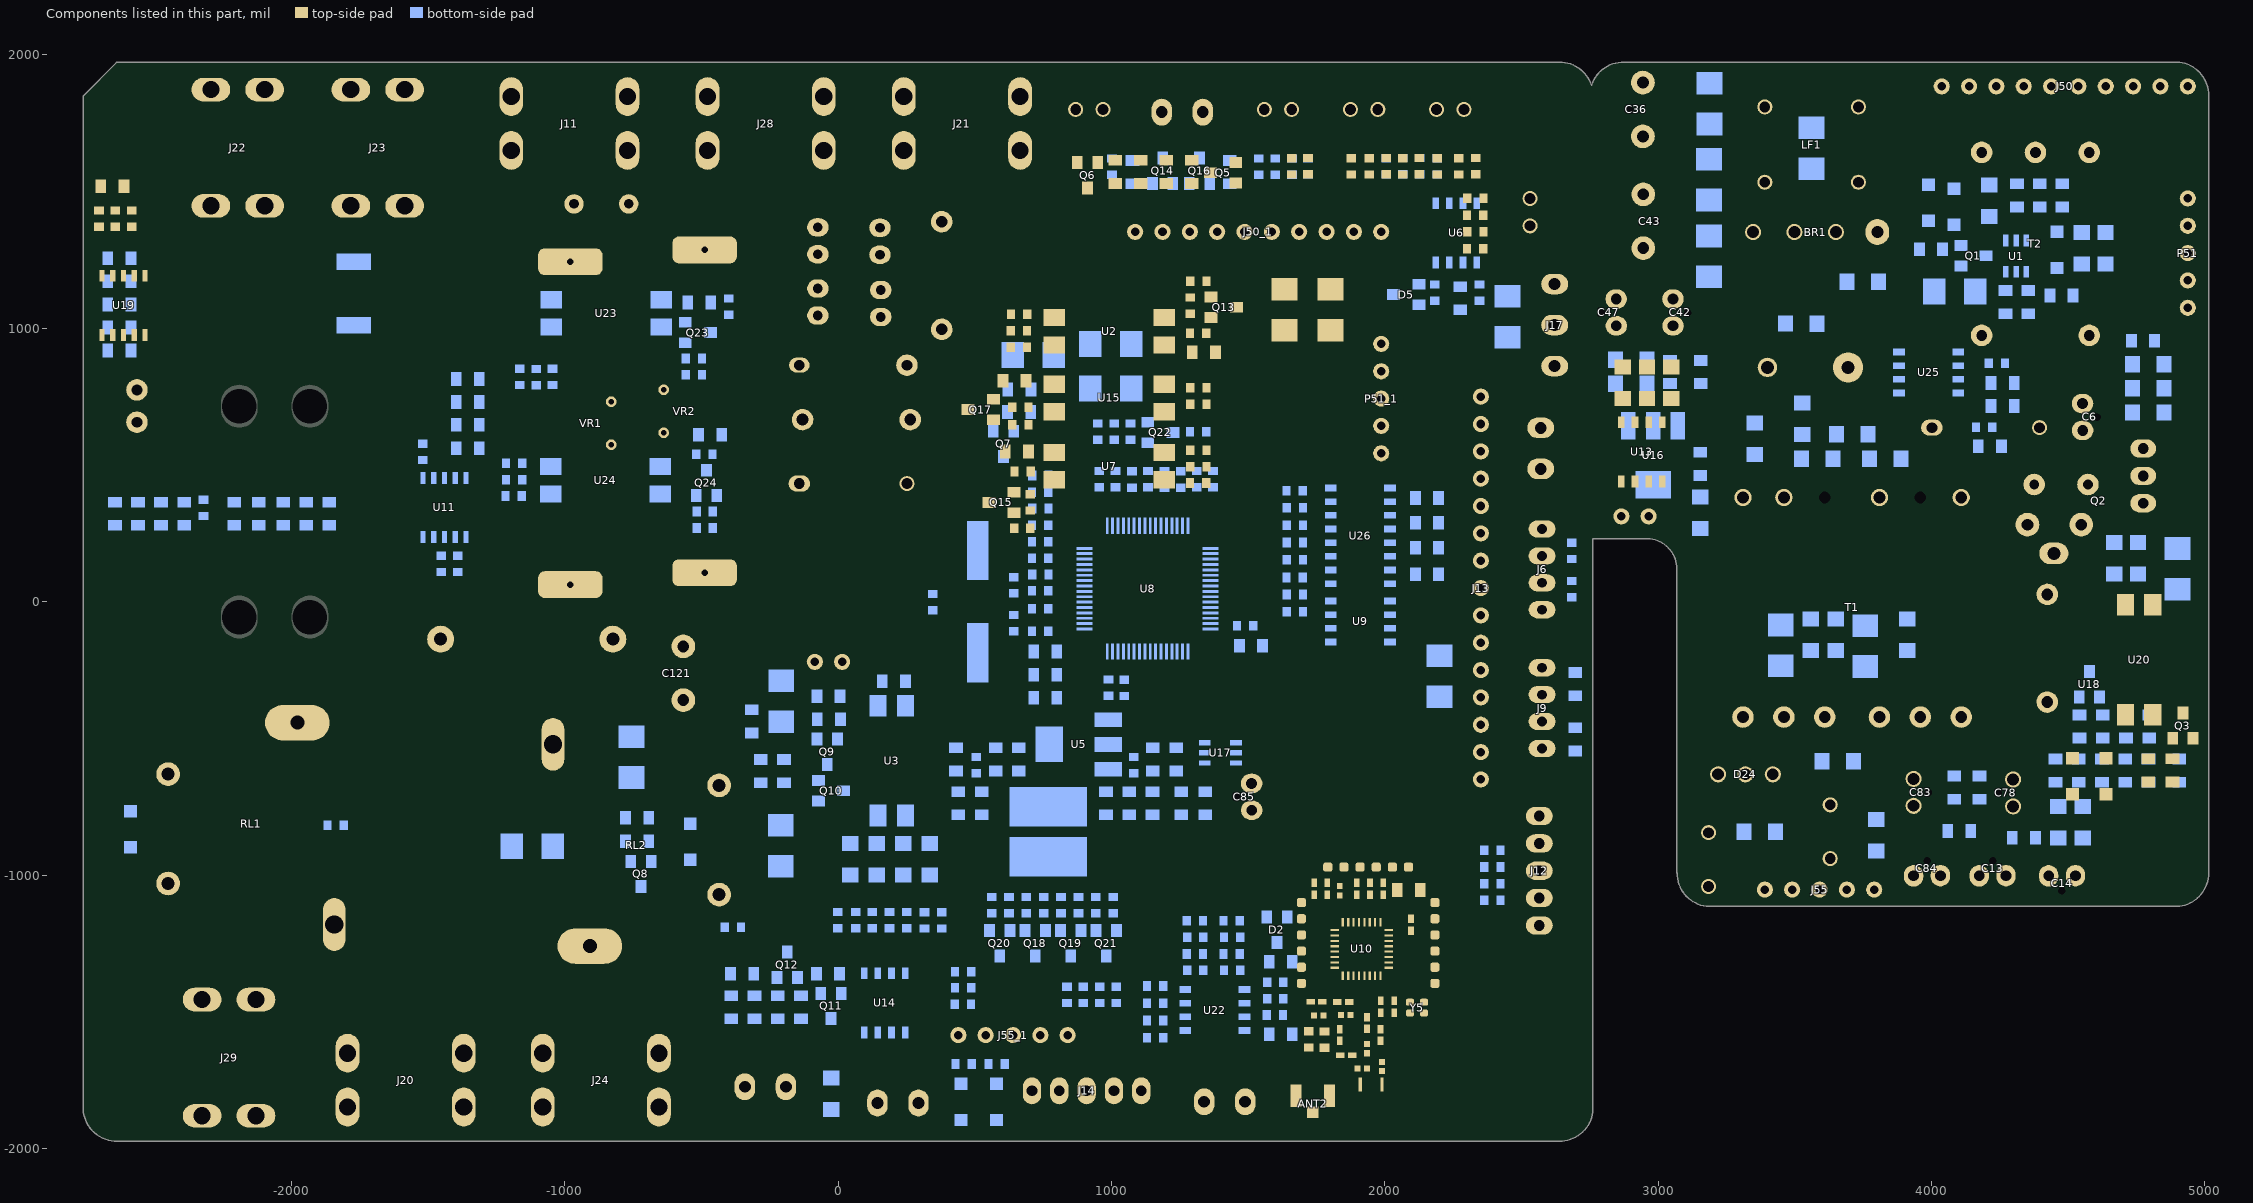
[diagram p0: the components of this part, seen from the top]
# Altium PCB MISC105418.PcbDoc (part 7 of 7)
Units mil, origin at the board's own origin, x right, y up, seen from the top; angles counter-clockwise.
Board outline 7774.32 x 3947.04 mil, 4 copper layers (Top Layer, 02, 03, Bottom Layer), stack 30.635 mil thick; 459 components, 285 nets, 1258 pads, 468 vias.
Unrouted connection lines stored in the file: 23.

## Polygon pours and split planes (outlines as drawn) (continued)
NetJP1_2 on Bottom Layer "NETJP1_2_L04_P172" (solid, remove dead copper, pour order 172): -2541,-310 -2257,-594 -1889,-594 -1857,-562 -1857,-403 -1888,-372 -2080,-372 -2121,-331 -2121,55 -2168,102 -2483,102 -2541,44
NetJP2_2 on Bottom Layer "NETJP2_2_L04_P170" (solid, remove dead copper, pour order 170): -2007,56 -2007,-198 -1950,-255 -1848,-255 -1727,-376 -1727,-585 -1651.67,-660.32 -1008.58,-660.33 -965,-616.74 -965,-433 -1084.99,-313 -1511,-313 -1632,-192 -1632,59 -1677,104 -1959,104
N2 on Bottom Layer "N2_L04_P198" (solid, remove dead copper, pour order 198): -534,1897 -534,1396 -610,1320 -610,1244 -597,1231 -353,1231 -248,1336 -37,1336 -6,1367 -6,1897 -39,1930 -501,1930
L-PLC on Bottom Layer "L-PLC_L04_P184" (solid, remove dead copper, pour order 184): -1193.8,1253.8 -1164,1224 -953,1224 -925,1252 -925,1464 -950,1489 -1168.58,1489 -1193.8,1462.76
L2 on Bottom Layer "L2_L04_P174" (solid, remove dead copper, pour order 174): -804,1389 -804,1534 -827,1557 -1240,1557 -1283,1600 -1283,1890 -1237,1936 -711,1936 -698,1923 -698,1387 -712,1373 -788,1373
ACL-OUT on Bottom Layer "ACL-OUT_L04_P146" (solid, remove dead copper, pour order 146): -1824,-1945 -1872,-1897 -1872,-1333 -1948,-1257 -1948,-1049 -1888,-989 -1394,-989 -1294,-1089 -1294,-1934 -1305,-1945
IP2 on Bottom Layer "IP2_L04_P132" (solid, remove dead copper, pour order 132): -1660,611 -1626,645 -1626,986 -1689,1049 -1803,1049 -2003,849 -2003,635 -1979,611
ACN-IN on Bottom Layer "ACN-IN_L04_P118" (solid, remove dead copper, pour order 118): -1552,1196 -1482,1266 -1482,1901 -1530,1949 -1839,1949 -1880,1908 -1880,1253 -1823,1196
ACN-OUT on Bottom Layer "ACN-OUT_L04_P116" (solid, remove dead copper, pour order 116): -1073,-1187 -1168,-1282 -1168,-1892 -1111,-1949 -620,-1949 -572,-1901 -572,-1275 -660,-1187
NetVR1_1 on Bottom Layer "NETVR1_1_L04_P044" (solid, remove dead copper, pour order 44): -1043,-198 -816,-198 -575,43 -374,43 -352,65 -352,134.25 -383.75,166 -1155,166 -1177,144 -1177,-64
NetC7_1 on Bottom Layer "NETC7_1_L04_P006" (solid, remove dead copper, pour order 6): 4783,187 4559,187 4494,252 4494,452 4519,477 4578,477 4610,445 4610,301.36 4666.35,245 4784,245 4791,238 4791,195
EARTH on Bottom Layer "EARTH_L04_P301" (solid, remove dead copper, pour order 301): 169,1538 195,1512 298,1512 321,1489 321,1372 347,1346 461,1346 481,1366 481,1472 510,1501 686,1501 735,1550 735,1921 704,1952 191,1952 169,1930
- on Top Layer "-_L01_P345" (solid, remove dead copper, pour order 345): 935,1901 935,872 -378,-441 -378,-1853 -301,-1930 2598,-1930 2700,-1828 2700,1851 2625,1926 960,1926
- on Top Layer "-_L01_P341" (solid, remove dead copper, pour order 341): 1541,-1443 1541,-1872 1620,-1951 1837,-1951 1879,-1909 1879,-1746 1900,-1725 2265,-1725 2286,-1704 2286,-1463 2246,-1423 2245,-1424 1560,-1424
- on Top Layer "-_L01_P339" (solid, remove dead copper, pour order 339): 1846,-1233 1846,-1315 1853,-1322 1924,-1322 1934,-1312 1934,-1239 1920,-1225 1854,-1225
EARTH on Top Layer "EARTH_L01_P331" (solid, remove dead copper, pour order 331): 169,1538 195,1512 298,1512 321,1489 321,1372 347,1346 461,1346 481,1366 481,1472 510,1501 686,1501 735,1550 735,1921 704,1952 191,1952 169,1930
EARTH on Top Layer "EARTH_L01_P323" (solid, remove dead copper, pour order 323): -2082,-1921 -2379,-1921 -2409,-1891 -2409,-1444 -2370,-1405 -2090,-1405 -2059,-1436 -2059,-1898
NetCX1_1 on Top Layer "Top Layer-NetCX1_1" (solid, remove dead copper, pour order 280): -7,1236 91,1334 205,1334 265,1274 265,1041 111,887 111,464 185,390 269,390 287.68,408.68 287.68,453.32 266,475 204,475 157,522 157,880 228,951 396,951 422,977 422,1012 398,1036 336,1036 318,1054 318,1293 205,1406 110,1406 9,1305 -96,1305 -111,1290 -111,1250 -97,1236
NetCX1_2 on Top Layer "NETCX1_2_L01_P277" (solid, remove dead copper, pour order 277): -104,392 -91,405 -91,679 54,824 54,1064 94,1104 195,1104 206,1115 206,1174 197,1183 74,1183 -28,1081 -97,1081 -122,1056 -122,1025 -45,948 -45,840 -192,693 -192,404 -180,392
L-3 on Top Layer "L-3_L01_P254" (solid, remove dead copper, pour order 254): 3406,1773 3511,1878 3950,1878 3982,1846 4061,1846 4073,1858 4073,1912 4050,1935 3435.74,1935 3352,1851.26 3352,1794 3373,1773
N on Top Layer "N_L01_P246" (solid, remove dead copper, pour order 246): 2827,1079 2879,1079 3012,1212 3620,1212 3696,1288 3696,1434 3769,1507 3769,1542 3746,1565 3719,1565 3617,1463 3617,1336 3571,1290 3034,1290 3006,1290 2862,1434 2862,1771 2905,1814 2940,1814 3001,1875 3001,1921 2978,1944 2856,1944 2811,1899 2811,1095
N2 on Top Layer "N2_L01_P234" (solid, remove dead copper, pour order 234): 4618,937 4788,1107 4788,1768 4644,1912 4626,1912 4613,1899 4613,1865 4739,1739 4739,1134 4616,1011 4561,1011 4539,989 4539,962 4564,937
NetCX3_1 on Top Layer "NETCX3_1_L01_P232" (solid, remove dead copper, pour order 232): 4148,723 4262,609 4413,609 4426,622 4426,647.39 4408.2,665.2 4293.8,665.2 4216,743 4216,993 4202,1007 4168.95,1007 4148,986.05
+311V on Top Layer "+311V_L01_P228" (solid, remove dead copper, pour order 228): 3758,1377 3758,1086 3635,963 3635,716 3926,425 4126,225 4370,225 4426,281 4426,433 4395,464 4004,464 3758.01,710 3758,953.34 3849,1044.34 3849,1381 3836.99,1393 3774,1393
NetJP2_2 on Top Layer "NETJP2_2_L01_P210" (solid, remove dead copper, pour order 210): -2007,56 -2007,-198 -1950,-255 -1848,-255 -1727,-376 -1727,-585 -1651.67,-660.32 -1008.58,-660.33 -965,-616.74 -965,-433 -1084.99,-313 -1511,-313 -1632,-192 -1632,59 -1677,104 -1959,104
NetJP1_2 on Top Layer "NETJP1_2_L01_P208" (solid, remove dead copper, pour order 208): -2541,-310 -2257,-594 -1889,-594 -1857,-562 -1857,-403 -1888,-372 -2080,-372 -2121,-331 -2121,55 -2168,102 -2483,102 -2541,44
NetVR1_1 on Top Layer "NETVR1_1_L01_P202" (solid, remove dead copper, pour order 202): -1043,-198 -824,-198 -605,21 -405,21 -345,81 -345,266 -398.01,319 -1105,319 -1177,247 -1177,-64
L2 on Top Layer "L2_L01_P176" (solid, remove dead copper, pour order 176): -804,1389 -804,1534 -827,1557 -1240,1557 -1283,1600 -1283,1890 -1237,1936 -711,1936 -698,1923 -698,1387 -712,1373 -788,1373
ACN-OUT on Top Layer "ACN-OUT_L01_P156" (solid, remove dead copper, pour order 156): -1073,-1187 -1168,-1282 -1168,-1892 -1111,-1949 -620,-1949 -572,-1901 -572,-1275 -660,-1187
ACL-OUT on Top Layer "ACL-OUT_L01_P154" (solid, remove dead copper, pour order 154): -1824,-1945 -1872,-1897 -1872,-1333 -1948,-1257 -1948,-1049 -1888,-989 -1394,-989 -1294,-1089 -1294,-1934 -1305,-1945
IP2 on Top Layer "IP2_L01_P138" (solid, remove dead copper, pour order 138): -1660,611 -1626,645 -1626,986 -1689,1049 -1798,1049 -2003,844 -2003,635 -1979,611
ACN-IN on Top Layer "ACN-IN_L01_P126" (solid, remove dead copper, pour order 126): -1552,1196 -1482,1266 -1482,1901 -1530,1949 -1839,1949 -1880,1908 -1880,1253 -1823,1196
ACL-IN on Top Layer "ACL-IN_L01_P120" (solid, remove dead copper, pour order 120): -2374,1900 -2374,1369 -2309,1304 -2309,665.39 -2281.61,638 -2154,638 -2127,665 -2127,901 -2003,1025 -2003,1892 -2050,1939 -2335,1939
L-PLC on Top Layer "L-PLC_L01_P291" (solid, remove dead copper, pour order 291): -1193.8,1253.8 -1164,1224 -953,1224 -925,1252 -925,1464 -950,1489 -1168.58,1489 -1193.8,1462.76
N2 on Top Layer "N2_L01_P293" (solid, remove dead copper, pour order 293): -534,1897 -534,1396 -610,1320 -610,1244 -597,1231 -353,1231 -248,1336 -37,1336 -6,1367 -6,1897 -39,1930 -501,1930
L-PLC on Top Layer "L-PLC_L01_P311" (solid, remove dead copper, pour order 311): -995,1055 -198,1055 -143,1110 -50,1110 -29,1131 -29,1159 -50,1180 -205,1180 -241,1144 -815.2,1144 -964.2,1293 -1157,1293 -1182,1268 -1182,1242
- on 03 "-_L03_P347" (solid, remove dead copper, pour order 347): 935,1901 935,760 -378,-553 -378,-1853 -301,-1930 2598,-1930 2700,-1828 2700,1851 2625,1926 960,1926
EARTH on 03 "EARTH_L03_P337" (solid, remove dead copper, pour order 337): 169,1538 195,1512 298,1512 321,1489 321,1372 347,1346 461,1346 481,1366 481,1472 510,1501 686,1501 735,1550 735,1921 704,1952 191,1952 169,1930
EARTH on 03 "EARTH_L03_P327" (solid, remove dead copper, pour order 327): -2082,-1921 -2379,-1921 -2409,-1891 -2409,-1444 -2370,-1405 -2090,-1405 -2059,-1436 -2059,-1898
L-3 on 03 "L-3_L03_P307" (solid, remove dead copper, pour order 307): 130,1061 130,920 228,822 731,822 1132,1223 1132,1379 1110,1401 1057.74,1401 1032,1375.26 1032,1249 706,923 623,923 288,923 235,976 235,1049 208,1076 145,1076
N-3 on 03 "N-3_L03_P305" (solid, remove dead copper, pour order 305): 42,823 77,858 77,1175 136,1234 224,1234 304,1154 810,1154 911,1255 911,1498 956,1543 1192,1543 1242,1493 1242,1310 1267,1285 1314,1285 1339,1310 1339,1524.86 1255.86,1608 898,1608 830,1540 830,1330 753,1253 326,1253 254,1325 115,1325 3,1213 3,982 -53,926 -199,926 -215,910 -215,839 -199,823
GND on 03 "03-GND" (solid, remove dead copper, pour order 270): 3236,275 3334,177 4084,177 4314,-53 4538,-53 4622,31 4622,497 4758,633 4758,1316.02 4484,1590 3963,1590 3808,1435 3319,1435 3236,1352
- on 03 "-_L03_P260" (solid, remove dead copper, pour order 260): 3955,-33 4147,-225 4845,-225 4974,-354 4974,-960 4858,-1076 3202.2,-1076 3105.2,-979 3105.2,-67.8 3140,-33
NetJP2_2 on 03 "NETJP2_2_L03_P214" (solid, remove dead copper, pour order 214): -2007,56 -2007,-198 -1950,-255 -1848,-255 -1727,-376 -1727,-585 -1651.67,-660.32 -1008.58,-660.33 -965,-616.74 -965,-433 -1084.99,-313 -1511,-313 -1632,-192 -1632,59 -1677,104 -1959,104
NetJP1_2 on 03 "NETJP1_2_L03_P212" (solid, remove dead copper, pour order 212): -2541,-310 -2257,-594 -1889,-594 -1857,-562 -1857,-403 -1888,-372 -2080,-372 -2121,-331 -2121,55 -2168,102 -2483,102 -2541,44
L2 on 03 "L2_L03_P180" (solid, remove dead copper, pour order 180): -804,1389 -804,1534 -827,1557 -1240,1557 -1283,1600 -1283,1890 -1237,1936 -711,1936 -698,1923 -698,1387 -712,1373 -788,1373
ACN-OUT on 03 "ACN-OUT_L03_P164" (solid, remove dead copper, pour order 164): -1073,-1187 -1168,-1282 -1168,-1892 -1111,-1949 -620,-1949 -572,-1901 -572,-1275 -660,-1187
ACL-OUT on 03 "ACL-OUT_L03_P162" (solid, remove dead copper, pour order 162): -1824,-1945 -1872,-1897 -1872,-1333 -1948,-1257 -1948,-1049 -1888,-989 -1394,-989 -1294,-1089 -1294,-1934 -1305,-1945
IP2 on 03 "IP2_L03_P134" (solid, remove dead copper, pour order 134): -1660,611 -1626,645 -1626,986 -1689,1049 -1798,1049 -2003,844 -2003,635 -1979,611
ACL-IN on 03 "ACL-IN_L03_P130" (solid, remove dead copper, pour order 130): -2374,1900 -2374,1369 -2309,1304 -2309,665.39 -2281.61,638 -2154,638 -2127,665 -2127,901 -2003,1025 -2003,1892 -2050,1939 -2335,1939
ACN-IN on 03 "ACN-IN_L03_P128" (solid, remove dead copper, pour order 128): -1552,1196 -1482,1266 -1482,1901 -1530,1949 -1839,1949 -1880,1908 -1880,1253 -1823,1196
L-PLC on 03 "L-PLC_L03_P283" (solid, remove dead copper, pour order 283): -1193.8,1253.8 -1164,1224 -953,1224 -925,1252 -925,1464 -950,1489 -1168.58,1489 -1193.8,1462.76
N2 on 03 "N2_L03_P285" (solid, remove dead copper, pour order 285): -534,1897 -534,1396 -610,1320 -610,1244 -597,1231 -353,1231 -248,1336 -37,1336 -6,1367 -6,1897 -39,1930 -501,1930
NetVR1_1 on 03 "NETVR1_1_L03_P297" (solid, remove dead copper, pour order 297): -1043,-198 -824,-198 -605,21 -405,21 -345,81 -345,266 -398.01,319 -1105,319 -1177,247 -1177,-64
- on 02 "-_L02_P349" (solid, remove dead copper, pour order 349): -993,625 -963,595 -827,595 -692,730 -408,730 -325,813 -325,999 -396,1070 -911,1070 -993,988
- on 02 "-_L02_P343" (solid, remove dead copper, pour order 343): 935,1901 935,760 -378,-553 -378,-1853 -301,-1930 2598,-1930 2700,-1828 2700,1851 2625,1926 960,1926
EARTH on 02 "EARTH_L02_P335" (solid, remove dead copper, pour order 335): 169,1538 195,1512 298,1512 321,1489 321,1372 347,1346 461,1346 481,1366 481,1472 510,1501 686,1501 735,1550 735,1921 704,1952 191,1952 169,1930
EARTH on 02 "EARTH_L02_P325" (solid, remove dead copper, pour order 325): -2082,-1921 -2379,-1921 -2409,-1891 -2409,-1444 -2370,-1405 -2090,-1405 -2059,-1436 -2059,-1898
NetJP2_2 on 02 "NETJP2_2_L02_P222" (solid, remove dead copper, pour order 222): -2007,56 -2007,-198 -1950,-255 -1848,-255 -1727,-376 -1727,-585 -1651.67,-660.32 -1008.58,-660.33 -965,-616.74 -965,-433 -1084.99,-313 -1511,-313 -1632,-192 -1632,59 -1677,104 -1959,104
NetJP1_2 on 02 "NETJP1_2_L02_P220" (solid, remove dead copper, pour order 220): -2541,-310 -2257,-594 -1889,-594 -1857,-562 -1857,-403 -1888,-372 -2080,-372 -2121,-331 -2121,55 -2168,102 -2483,102 -2541,44
GND on 02 "02-GND" (solid, remove dead copper, pour order 271): 3236,275 3334,177 4084,177 4314,-53 4538,-53 4622,31 4622,497 4758,633 4758,911 4198,1471 4109,1560 3933,1560 3808,1435 3319,1435 3236,1352
- on 02 "-_L02_P262" (solid, remove dead copper, pour order 262): 3955,-33 4147,-225 4845,-225 4974,-354 4974,-960 4858,-1076 3202.2,-1076 3105.2,-979 3105.2,-67.8 3140,-33
L2 on 02 "L2_L02_P178" (solid, remove dead copper, pour order 178): -804,1389 -804,1534 -827,1557 -1240,1557 -1283,1600 -1283,1890 -1237,1936 -711,1936 -698,1923 -698,1387 -712,1373 -788,1373
ACN-OUT on 02 "ACN-OUT_L02_P160" (solid, remove dead copper, pour order 160): -1073,-1187 -1168,-1282 -1168,-1892 -1111,-1949 -620,-1949 -572,-1901 -572,-1275 -660,-1187
ACL-OUT on 02 "ACL-OUT_L02_P158" (solid, remove dead copper, pour order 158): -1824,-1945 -1872,-1897 -1872,-1333 -1948,-1257 -1948,-1049 -1888,-989 -1394,-989 -1294,-1089 -1294,-1934 -1305,-1945
ACN-IN on 02 "ACN-IN_L02_P140" (solid, remove dead copper, pour order 140): -1552,1196 -1482,1266 -1482,1901 -1530,1949 -1839,1949 -1880,1908 -1880,1253 -1823,1196
IP2 on 02 "IP2_L02_P136" (solid, remove dead copper, pour order 136): -1660,611 -1626,645 -1626,986 -1689,1049 -1798,1049 -2003,844 -2003,635 -1979,611
ACL-IN on 02 "ACL-IN_L02_P122" (solid, remove dead copper, pour order 122): -2382,1902 -2382,1371 -2317,1306 -2317,667.39 -2289.61,640 -2162,640 -2135,667 -2135,903 -2011,1027 -2011,1894 -2058,1941 -2343,1941
L-PLC on 02 "L-PLC_L02_P287" (solid, remove dead copper, pour order 287): -1193.8,1253.8 -1164,1224 -953,1224 -925,1252 -925,1464 -950,1489 -1168.58,1489 -1193.8,1462.76
N2 on 02 "N2_L02_P289" (solid, remove dead copper, pour order 289): -534,1897 -534,1396 -610,1320 -610,1244 -597,1231 -353,1231 -248,1336 -37,1336 -6,1367 -6,1897 -39,1930 -501,1930
NetVR1_1 on 02 "NETVR1_1_L02_P295" (solid, remove dead copper, pour order 295): -1043,-198 -824,-198 -605,21 -405,21 -345,81 -345,266 -398.01,319 -1105,319 -1177,247 -1177,-64
ACL-OUT on Bottom Solder "ACL-OUT_L02_P158" (solid): -1824,-1945 -1872,-1897 -1872,-1333 -1948,-1257 -1948,-1049 -1888,-989 -1394,-989 -1294,-1089 -1294,-1934 -1305,-1945
ACN-OUT on Bottom Solder "ACN-OUT_L02_P160" (solid): -1073,-1187 -1168,-1282 -1168,-1892 -1111,-1949 -620,-1949 -572,-1901 -572,-1275 -660,-1187
EARTH on Bottom Solder "EARTH_L02_P325" (solid): -2082,-1921 -2379,-1921 -2409,-1891 -2409,-1444 -2370,-1405 -2090,-1405 -2059,-1436 -2059,-1898
NetVR1_1 on Bottom Solder "NETVR1_1_L04_P044" (solid): -1043,-198 -816,-198 -575,43 -374,43 -352,65 -352,134.25 -383.75,166 -1155,166 -1177,144 -1177,-64
NetJP2_2 on Bottom Solder "NETJP2_2_L04_P170" (solid): -2007,56 -2007,-198 -1950,-255 -1848,-255 -1727,-376 -1727,-585 -1651.67,-660.32 -1008.58,-660.33 -965,-616.74 -965,-433 -1084.99,-313 -1511,-313 -1632,-192 -1632,59 -1677,104 -1959,104
NetJP1_2 on Bottom Solder "NETJP1_2_L04_P172" (solid): -2541,-310 -2257,-594 -1889,-594 -1857,-562 -1857,-403 -1888,-372 -2080,-372 -2121,-331 -2121,55 -2168,102 -2483,102 -2541,44
ACN-IN on Bottom Solder "ACN-IN_L04_P118" (solid): -1552,1196 -1482,1266 -1482,1901 -1530,1949 -1839,1949 -1880,1908 -1880,1253 -1823,1196
IP2 on Bottom Solder "IP2_L04_P132" (solid): -1660,611 -1626,645 -1626,986 -1689,1049 -1803,1049 -2003,849 -2003,635 -1979,611
L2 on Bottom Solder "L2_L04_P174" (solid): -804,1389 -804,1534 -827,1557 -1240,1557 -1283,1600 -1283,1890 -1237,1936 -711,1936 -698,1923 -698,1387 -712,1373 -788,1373
L-PLC on Bottom Solder "L-PLC_L04_P184" (solid): -1193.8,1253.8 -1164,1224 -953,1224 -925,1252 -925,1464 -950,1489 -1168.58,1489 -1193.8,1462.76
N2 on Bottom Solder "N2_L04_P198" (solid): -534,1897 -534,1396 -610,1320 -610,1244 -597,1231 -353,1231 -248,1336 -37,1336 -6,1367 -6,1897 -39,1930 -501,1930
ACL-IN on Bottom Solder "ACL-IN_L04_P224" (solid): -2382,1902 -2382,1371 -2382,687 -2330,635 -2157,635 -2135,657 -2135,903 -2011,1027 -2011,1894 -2058,1941 -2343,1941
EARTH on Bottom Solder "EARTH_L04_P301" (solid): 169,1538 195,1512 298,1512 321,1489 321,1372 347,1346 461,1346 481,1366 481,1472 510,1501 686,1501 735,1550 735,1921 704,1952 191,1952 169,1930

## Keep-outs
Keep-Out Layer:
  lines w7.87: 2756.09,234.5 2756.09,1859.5
  lines w10: -2637.91,-1968.5 2637.09,-1968.5 ccw(c2639.05,-1850.39) 2756.09,-1866.21 2756.09,1859.5 ; -2636.91,-1968.49 cw(c-2638.86,-1850.39) -2755.91,-1866.21 -2755.91,1847.97 -2636.53,1968.5 2637.91,1968.5 ; 2636.91,1968.49 cw(c2638.86,1850.39) 2755.91,1866.21 ; 2755.91,-1859.5 2755.91,1866.21 ; 2756.09,235.5 2971.09,235.5 cw(c2955.28,118.46) 3073.37,116.5 ; 2874.91,1968.49 ccw(c2872.95,1850.39) 2755.91,1866.21 ; 2875.09,1968.5 4906.09,1968.5 cw(c4890.28,1851.46) 5008.37,1849.5 ; 3073.28,-990.5 3073.28,118.46 ; 3073.82,-990.5 ccw(c3191.91,-992.45) 3176.09,-1109.5 4906.09,-1109.5 ccw(c4890.28,-992.45) 5008.37,-990.5 ; 5007.98,-990.5 5007.98,1851.46
  lines w98.43: -2061.99,-207 -2062,82 ; -2061.99,568 -2062,857

## Other copper
Top Layer:
  pour cut-out: 2268,619 2286,601 2408,601 2431,624 2431,802 2402,831 2286,831 2268,813
  pour cut-out: 2006.98,1445 2046,1406.02 2046,1295.8 2011.21,1261.01 1086.75,1261 1061,1286.75 1061,1428 1078,1445
02:
  pour cut-out: -422.14,-850 -379,-850 -128,-1101 -128,-1930 -149,-1951 -174,-1926 -435,-1926 -465,-1896 -465,-1819
  pour cut-out: 3358,1448 3402,1404 3402,1300 3443,1259 3831,1259 3892,1320 3892,1529 3916,1553
  pour cut-out: 4296.35,428.5 ccw(c4375.09,428.5) 4375.09,349.76 ccw(c4375.09,428.5) 4453.83,428.5 ccw(c4375.09,428.5) 4375.09,507.24 ccw(c4375.09,428.5)
  pour cut-out: 4271.93,281.5 ccw(c4350.67,281.5) 4350.67,202.76 ccw(c4350.67,281.5) 4429.41,281.5 ccw(c4350.67,281.5) 4350.67,360.24 ccw(c4350.67,281.5)
  pour cut-out: 4029.57,381.08 ccw(c4108.31,381.08) 4108.31,302.34 ccw(c4108.31,381.08) 4187.05,381.08 ccw(c4108.31,381.08) 4108.31,459.82 ccw(c4108.31,381.08)
  pour cut-out: 3922.35,636.5 ccw(c4001.09,636.5) 4001.09,557.76 ccw(c4001.09,636.5) 4079.83,636.5 ccw(c4001.09,636.5) 4001.09,715.24 ccw(c4001.09,636.5)
  pour cut-out: 4497.96,974 ccw(c4576.7,974) 4576.7,895.26 ccw(c4576.7,974) 4655.44,974 ccw(c4576.7,974) 4576.7,1052.74 ccw(c4576.7,974)
  pour cut-out: 4104.26,974 ccw(c4183,974) 4183,895.26 ccw(c4183,974) 4261.74,974 ccw(c4183,974) 4183,1052.74 ccw(c4183,974)
  pour cut-out: 3615.9,857 ccw(c3694.64,857) 3694.64,778.26 ccw(c3694.64,857) 3773.38,857 ccw(c3694.64,857) 3694.64,935.74 ccw(c3694.64,857)
03:
  pour cut-out: 2041,1445 2046,1440 2046,1315.6 2011,1280.6 1379.48,1280.6 1347.2,1312.89 1347.2,1422.2 1370,1445
  pour cut-out: 1445,1282 926,763 916,763 916,959 1234,1277 1312.11,1277 1344.11,1309 1420,1309 1434,1295
  pour cut-out: 885,1657 1327,1657 1445,1539 1445,1282 1378.08,1282 1347.2,1312.89 1347.2,1520.8 1256,1612 899,1612 853,1658 853,1659
  pour cut-out: 3383,1447 3397,1433 3397,1297 3448,1246 3840,1246 3907.41,1313.41 3907.41,1534.59 3901,1541
Bottom Layer:
  rectangle net D5V: 626,-715 1091,-657
  rectangle net D5V: 416,-823 911,-744.83
  rectangle net D3.3V: 794,-553 1043,-491
  rectangle net D5V: 938,-715 1091,-630

## Silkscreen, mask and mechanical layers (free items; w line width, h text height)
Mechanical 6:
  circle w4.92: c-2598.43,1771.65 r98.43
  circle w4.92: c-2598.43,-1771.65 r98.43
  circle w4.92: c2598.43,-1771.65 r98.43
  circle w4.92: c2598.43,1771.65 r98.43
  lines w7.87: 887.81,-1534.74 890.81,-1537.74 ; 2756.09,234.5 2756.09,1859.5 ; 3838.09,-1002.5 3841.09,-1005.5 ; -194.19,-297.74 -194.19,1327.26 -194.19,-297.74 ; -134.28,-272.24 64.72,-272.24 64.72,-170.24 -134.28,-170.24 -134.28,-272.24 ; 390.72,-1639.24 390.72,-1537.24 892.72,-1537.24 892.72,-1639.24 390.72,-1639.24 ; 1037.72,1303.38 2036.81,1303.38 2036.81,1405.38 1037.72,1405.38 1037.72,1303.38 ; 1936.72,491.76 2038.72,491.76 2038.72,992.76 1936.72,992.76 1936.72,491.76 ; 2816,260 2816,362 3015,362 3015,260 2816,260 ; 3341,-1107 3843,-1107 3843,-1005 3341,-1005 3341,-1107 ; 3988,1835.62 3988,1937.62 4987.09,1937.62 4987.09,1835.62 3988,1835.62 ; 4887,1024 4887,1525 4989,1525 4989,1024 4887,1024
  lines w10: -194.38,1333.97 cw(c-77.33,1318.15) -75.38,1436.24 ; -75.19,1436.26 1955.81,1436.26 cw(c1939.99,1319.21) 2058.09,1317.26 ; 123,-1522.74 123,-413.79 ; 123.09,-415.74 ccw(c4.99,-413.79) 20.81,-296.74 ; 123.53,-1522.74 ccw(c241.63,-1524.69) 225.81,-1641.74 ; 2057.7,-1522.74 2057.7,1319.21 ; 2058.09,-1522.74 cw(c1939.99,-1524.69) 1955.81,-1641.74 ; 2755.91,1866.21 cw(c2872.95,1850.39) 2874.91,1968.49 ; 2756.09,235.5 2971.09,235.5 cw(c2955.28,118.46) 3073.37,116.5 ; 2875.09,1968.5 4906.09,1968.5 cw(c4890.28,1851.46) 5008.37,1849.5 ; 3073.28,-990.5 3073.28,118.46 ; 3073.82,-990.5 ccw(c3191.91,-992.45) 3176.09,-1109.5 4906.09,-1109.5 ccw(c4890.28,-992.45) 5008.37,-990.5 ; 5007.98,-990.5 5007.98,1851.46 ; 20.81,-296.74 -194.19,-296.74 20.81,-296.74 ; 225.81,-1641.74 1955.81,-1641.74 ; 225.81,-1641.74 1955.81,-1641.74
  lines w40: -2769,-765 -1248,-765 -291,192 -291,1466
  lines w118.11: -2066,457 -2066,872 -1941,997 -1941,1901 ; -502,-1888.54 -502,-408 149,243 324,418 324,680 324,864 502,1042 502,1193 637,1328 793,1484 793,1917 ; 3162.09,73.5 3983.09,73.5 4205.09,-148.5 4930.09,-148.5 ; 3170.09,829.5 3170.09,593.5 3175.09,498.5 ; 3171,834 3171,874 3502.5,1205.5 3759.09,1205.5 3890.09,1074.5 3890.09,916.5 3890.09,494.5 ; 4834,1549 4834,1002 4883,953 4955,953